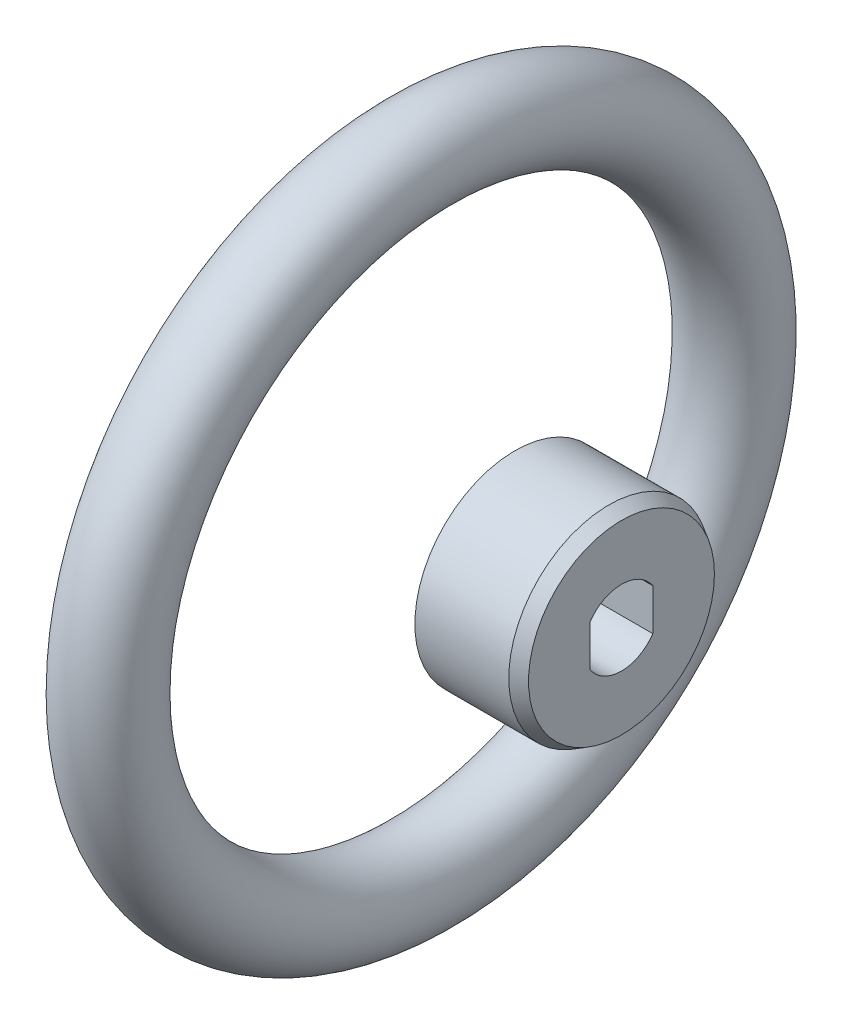
SolidWorks part; units mm, degrees
ref_plane "Front Plane" through (0, 0, 0) normal (0, 0, 1) x (1, 0, 0)
ref_plane "Top Plane" through (0, 0, 0) normal (0, 1, 0) x (1, 0, 0)
ref_plane "Right Plane" through (0, 0, 0) normal (1, 0, 0) x (0, 0, -1)
sketch "Sketch1" plane through (0, 0, 0) normal (0, 0, 1) x (1, 0, 0)
  circle A0 centre (0, 0) radius 7
  dimension "D1" = 14
sketch "Sketch2" plane through (0, 0, 0) normal (1, 0, 0) x (0, 0, -1)
  circle A0 centre (0, -50) radius 50
  dimension "D1" = 100
  dimension "D2" = 50
sweep "Sweep1" add profiles "Sketch1" path "Sketch2"
ref_plane "Plane1" through (32, 0, 0) normal (1, 0, 0) x (0, 0, -1)
sketch "Sketch3" plane through (32, 0, 0) normal (1, 0, 0) x (0, 0, -1)
  circle A0 centre (0, -50) radius 16
  dimension "D1" = 32
extrude "Boss-Extrude1" add sketch "Sketch3" against normal blind 17 separate body
chamfer "Chamfer1" distance 2 angle 30 1 edges at (32, -50, -16)
ref_plane "Plane2" through (-7.2224, -12.5096, 0) normal (0.5, 0.866, 0) x (-0.866, 0.5, 0)
sketch "Sketch5" plane through (-7.2224, -12.5096, 0) normal (0.5, 0.866, 0) x (-0.866, 0.5, 0)
  line L0 (-32.8675, 19.0921) -> (-32.8675, -23.2254)
ref_plane "Plane3" through (-3.8509, -3.8509, 0) normal (0.7071, 0.7071, 0) x (-0.7071, 0.7071, 0)
sketch "Sketch6" plane through (32, 0, 0) normal (1, 0, 0) x (0, 0, -1)
  line L0 (-5, -46.6834) -> (-5, -53.3166)
  line L1 (5, -46.6834) -> (5, -53.3166)
  arc A0 (5, -46.6834) -> (-5, -46.6834) centre (0, -50) ccw
  arc A1 (-5, -53.3166) -> (5, -53.3166) centre (0, -50) ccw
  dimension "D1" = 12
  dimension "D2" = 5
  dimension "D3" = 5
extrude "Cut-Extrude1" cut sketch "Sketch6" against normal through all
